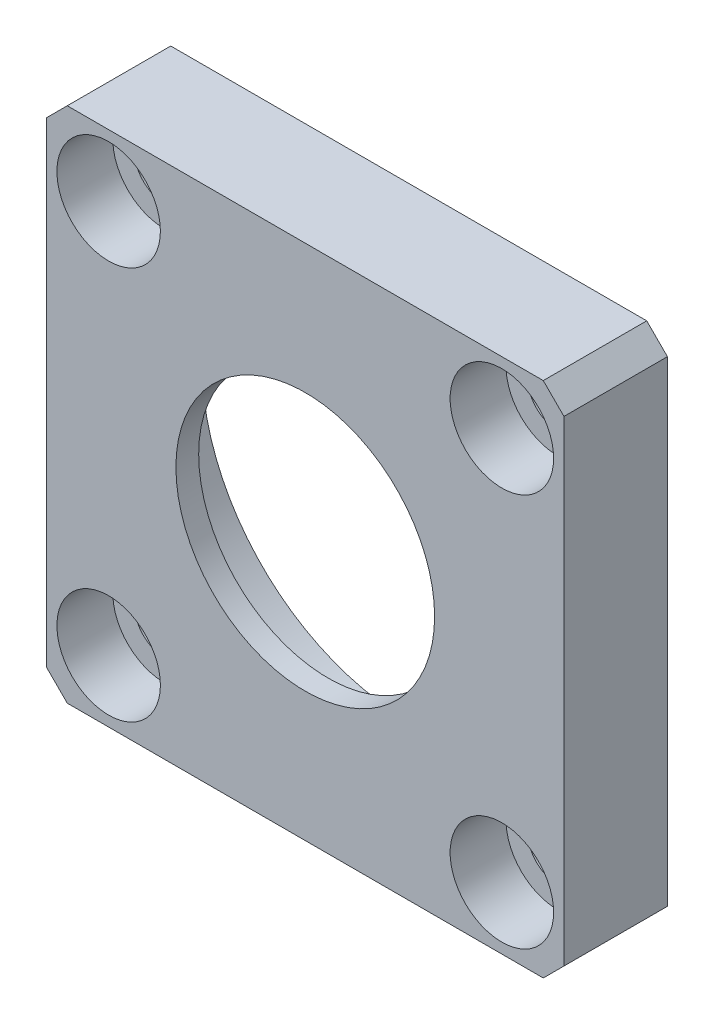
SolidWorks part; units mm, degrees
material "6061Al"
ref_plane "前视基准面" through (0, 0, 0) normal (0, 0, 1) x (1, 0, 0)
ref_plane "上视基准面" through (0, 0, 0) normal (0, 1, 0) x (1, 0, 0)
ref_plane "右视基准面" through (0, 0, 0) normal (1, 0, 0) x (0, 0, -1)
sketch "草图1" plane through (0, 0, 0) normal (0, 0, 1) x (1, 0, 0)
  line L1 (-25, -25) -> (25, -25)
  line L2 (-25, -25) -> (-25, 25)
  line L3 (-25, 25) -> (25, 25)
  line L4 (25, -25) -> (25, 25)
  line L5 (-25, -25) -> (25, 25) construction
  line L6 (-25, 25) -> (25, -25) construction
  point P0 (0, 0)
  dimension "D1" = 50
  dimension "D2" = 50
extrude "凸台-拉伸1" add sketch "草图1" along normal mid plane 10
sketch "草图2" plane through (0, 0, 5) normal (0, 0, 1) x (1, 0, 0)
  circle A0 centre (0, 0) radius 20
  dimension "D1" = 40
extrude "切除-拉伸1" cut sketch "草图2" against normal through all
hole_wizard "M5 六角凹头螺钉的柱形沉头孔1" positions "草图6" profile "草图5" counterbore size "M5" standard "ISO" end condition through all
sketch "草图6" plane through (0, 0, 5) normal (0, 0, 1) x (1, 0, 0)
  line L1 (-19, -19) -> (19, -19)
  line L2 (-19, -19) -> (-19, 19)
  line L3 (-19, 19) -> (19, 19)
  line L4 (19, -19) -> (19, 19)
  line L5 (-19, -19) -> (19, 19) construction
  line L6 (-19, 19) -> (19, -19) construction
  line L7 (-25, 25) -> (-25, -25) construction
  point P0 (-19, 19)
  point P4 (19, 19)
  point P7 (-19, -19)
  point P9 (19, -19)
  dimension "D1" = 6
sketch "草图5" plane through (-19, 19, 5) normal (1, 0, 0) x (0, -1, 0)
  line L0 (0, 0) -> (0, 10)
  line L1 (0, 10) -> (2.9, 10)
  line L3 (2.9, 10) -> (2.9, 5.4)
  line L4 (2.9, 5.4) -> (5, 5.4)
  line L5 (5, 5.4) -> (5, 0)
  line L7 (5, 0) -> (0, 0)
  line L11 (0, -6.35) -> (0, 107.95) construction
  dimension "通孔孔直径" = 5.8
  dimension "通孔孔深度" = 10
  dimension "柱形沉头孔直径" = 10
  dimension "柱形沉头孔深度" = 5.4
chamfer "倒角1" distance 2 angle 45 4 edges at (-25, -25, 0) (25, -25, 0) (25, 25, 0) (-25, 25, 0)
sketch "草图7" plane through (0, 0, 5) normal (0, 0, 1) x (1, 0, 0)
  circle A0 centre (0, 0) radius 20 construction
  circle A1 centre (0, 0) radius 20
  circle A2 centre (0, 0) radius 12.5
  dimension "D1" = 25
extrude "凸台-拉伸2" add sketch "草图7" against normal blind 2.2
